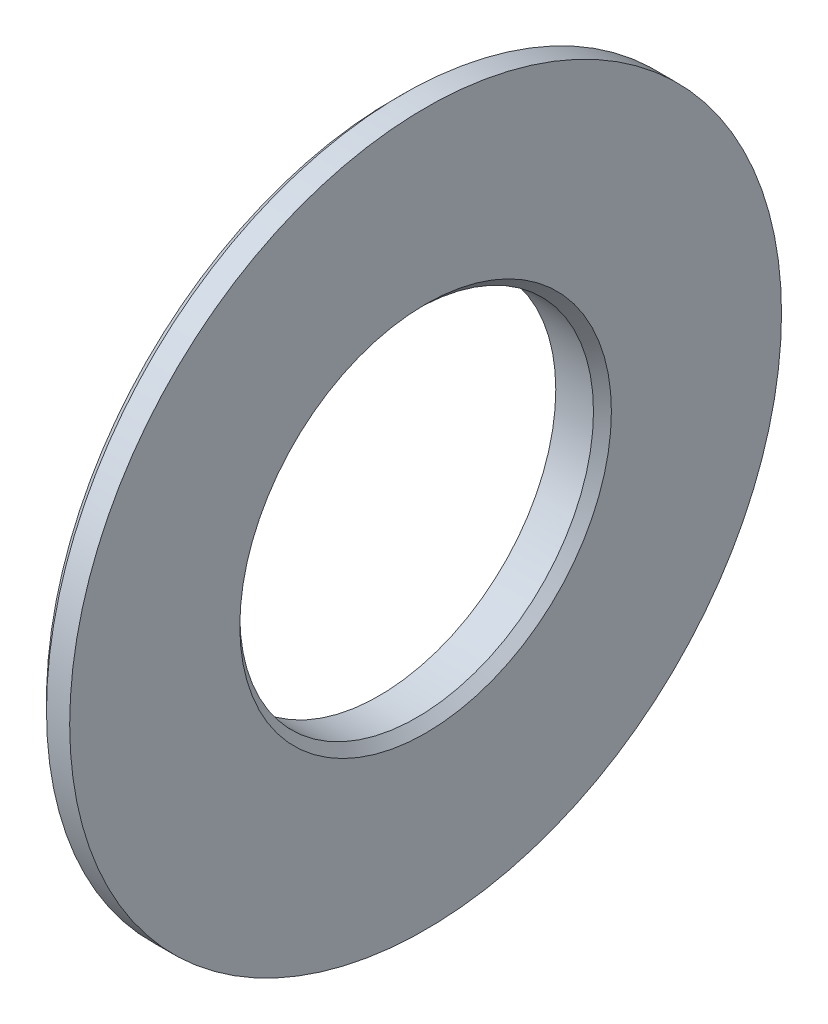
SolidWorks part; units mm, degrees
ref_plane "前视基准面" through (0, 0, 0) normal (0, 0, 1) x (1, 0, 0)
ref_plane "上视基准面" through (0, 0, 0) normal (0, 1, 0) x (1, 0, 0)
ref_plane "右视基准面" through (0, 0, 0) normal (1, 0, 0) x (0, 0, -1)
sketch "草图1" plane through (0, 0, 0) normal (0, 0, 1) x (1, 0, 0)
  line L1 (4.0254, -22.417) -> (27.1434, -22.417) construction
  line L2 (6.5034, -2.667) -> (6.5034, 2.333)
  line L3 (6.5034, 2.333) -> (8.1232, 2.333)
  line L4 (8.1232, 2.333) -> (8.1232, 17.333)
  line L5 (8.1232, 17.333) -> (11.7134, 17.333)
  line L6 (11.7134, 17.333) -> (11.7134, -2.667)
  line L7 (11.7134, -2.667) -> (6.5034, -2.667)
  dimension "D1" = 5.21
  dimension "D2" = 5
  dimension "D3" = 20
  dimension "D4" = 19.75
revolve "旋转1" add sketch "草图1" angle 360 about L1
chamfer "倒角1" distance 1 angle 45 1 edges at (8.1232, -22.417, 39.75)
chamfer "倒角2" distance 1 angle 45 1 edges at (11.7134, -22.417, 19.75)
